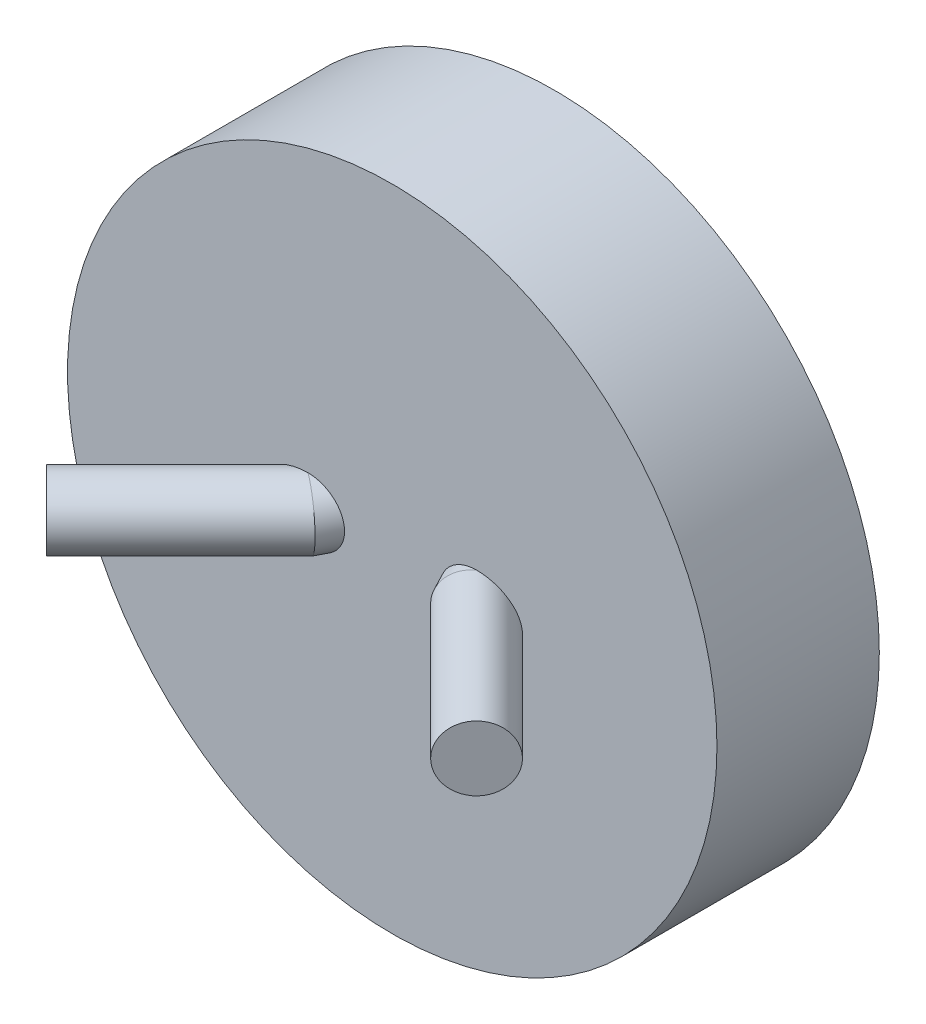
SolidWorks part; units mm, degrees
ref_plane "Front Plane" through (0, 0, 0) normal (0, 0, 1) x (1, 0, 0)
ref_plane "Top Plane" through (0, 0, 0) normal (0, 1, 0) x (1, 0, 0)
ref_plane "Right Plane" through (0, 0, 0) normal (1, 0, 0) x (0, 0, -1)
sketch "Sketch1" plane through (0, 0, 0) normal (0, 0, 1) x (1, 0, 0)
  circle A0 centre (0, 0) radius 10
  dimension "D1" = 20
extrude "Boss-Extrude1" add sketch "Sketch1" along normal mid plane 5
sketch "Sketch3" plane through (0, 0, 0) normal (0, 1, 0) x (1, 0, 0)
  line L0 (0, 2.5) -> (0, -2.5) construction
  line L1 (-10, -2.5) -> (10, -2.5) construction
  line L2 (0, -2.5) -> (-4.0781, -6.5781) construction
  line L3 (0, -2.5) -> (4.0781, -6.5781) construction
  line L4 (0, 2.5) -> (-4.0781, 6.5781)
  line L5 (0, 2.5) -> (3.5355, 6.0355)
  line L6 (10, 2.5) -> (-10, 2.5) construction
  dimension "D1" = 45
  dimension "D2" = 45
  dimension "D3" = 45
  dimension "D4" = 45
  dimension "D5" = 5
ref_plane "Plane1" through (3.5355, 0, -6.0355) normal (0.7071, 0, -0.7071) x (-0.7071, 0, -0.7071)
sketch "Sketch5" plane through (3.5355, 0, -6.0355) normal (0.7071, 0, -0.7071) x (-0.7071, 0, -0.7071)
  line L0 (0, 0) -> (5.7674, 0) construction
  line L1 (0, 0) -> (-3.5355, 0) construction
  circle A0 centre (0, 0) radius 1
  dimension "D1" = 2
sweep "Sweep1" add profiles "Sketch5" path "Sketch3"
sketch "Sketch6" plane through (0, 0, 0) normal (0, 1, 0) x (1, 0, 0)
  line L0 (3.5355, 6.0355) -> (0, 2.5) construction
  line L1 (4.2426, 5.3284) -> (2.8284, 6.7426) construction
  line L2 (10, 2.5) -> (-10, 2.5) construction
  line L3 (0, 2.5) -> (-4.0781, 6.5781) construction
  line L4 (-3.371, 7.2852) -> (-4.7852, 5.871) construction
  line L5 (0, 2.5) -> (0, -2.5) construction
  line L6 (-10, -2.5) -> (10, -2.5) construction
  line L7 (0, 2.5) -> (2.5958, -2.5) construction
  line L8 (2.5958, -2.5) -> (6.5682, -6.4724) construction
  line L9 (0, 2.5) -> (-2.5958, -2.5) construction
  line L10 (-2.5958, -2.5) -> (-6.6193, -6.5234) construction
  line L11 (-2.5958, -2.5) -> (3.2479, -8.3437)
  line L12 (2.5958, -2.5) -> (-3.2425, -8.3384)
  dimension "D1" = 1.7
  dimension "D2" = 1.7
  dimension "D3" = 45
  dimension "D4" = 45
ref_plane "Plane2" through (-6.6193, 0, 6.5234) normal (-0.7071, 0, 0.7071) x (0.7071, 0, 0.7071)
sketch "Sketch7" plane through (-6.6193, 0, 6.5234) normal (-0.7071, 0, 0.7071) x (0.7071, 0, 0.7071)
  circle A0 centre (0, 0) radius 1
  dimension "D1" = 2
sketch "Sketch8" plane through (0, 0, 0) normal (0, 1, 0) x (1, 0, 0)
  line L0 (3.5355, 6.0355) -> (0, 2.5) construction
  line L1 (0, 2.5) -> (-2.5958, -2.5) construction
  line L2 (-2.5958, -2.5) -> (-6.6193, -6.5234) construction
  line L3 (3.5355, 6.0355) -> (0, 2.5)
  line L4 (0, 2.5) -> (-2.5958, -2.5)
  line L5 (-2.5958, -2.5) -> (-6.6193, -6.5234)
sweep "Sweep2" add profiles "Sketch7" path "Sketch8"
mirror "Mirror1" about plane through (0, 0, 0) normal (1, 0, 0) of "Sweep2"
